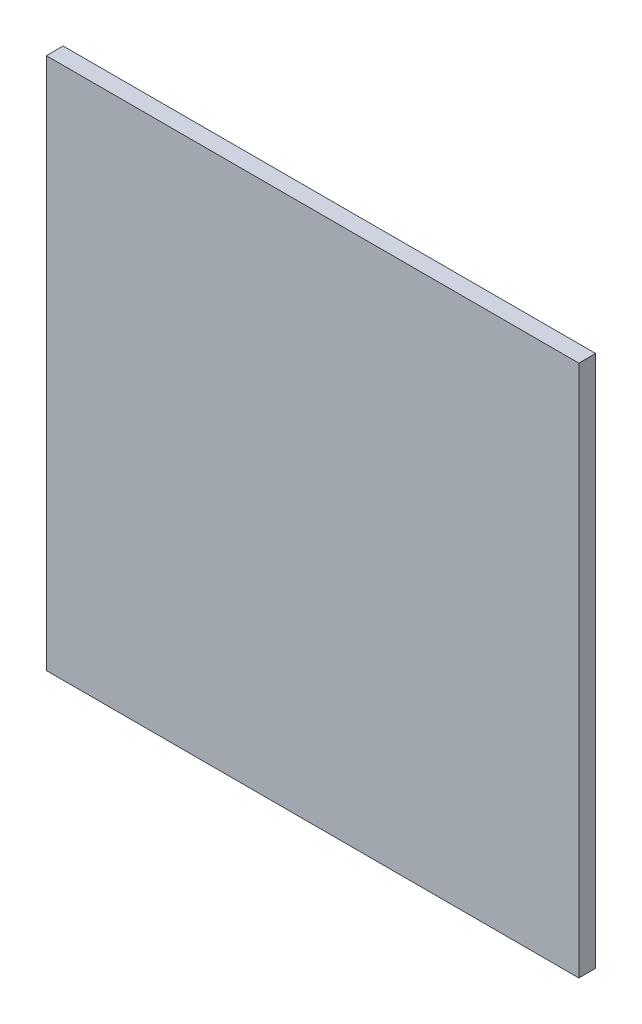
from build123d import *

# Parameters (mm, degrees)
SKETCH1_W           = 254
SKETCH1_H           = 254
BOSS_EXTRUDE1_DEPTH = 4


with BuildPart() as part:
    # Sketch1 → Boss-Extrude1 (new, symmetric)
    with BuildSketch(Plane.XY):
        Rectangle(SKETCH1_W, SKETCH1_H)
    extrude(amount=BOSS_EXTRUDE1_DEPTH, both=True)


solid = part.part
